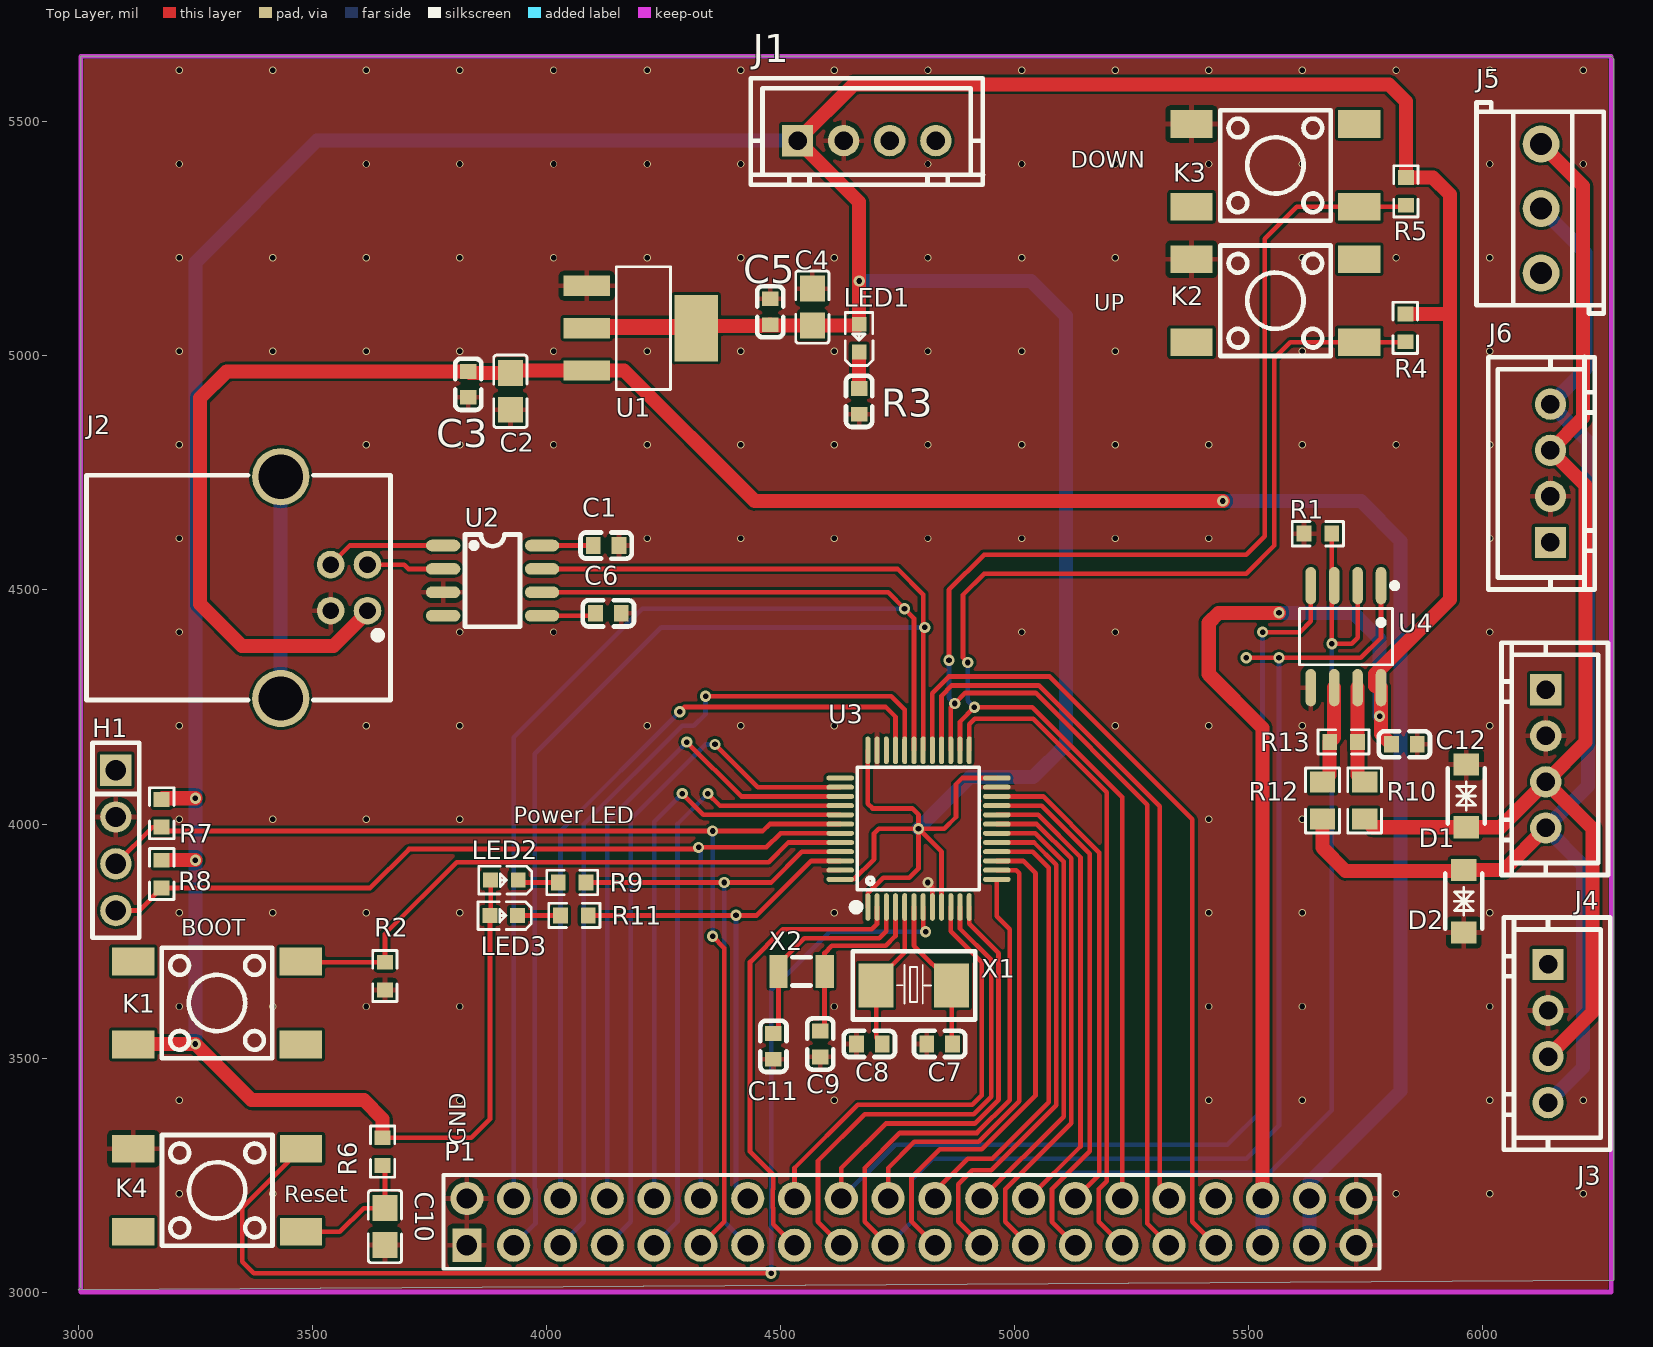
[diagram p0: Top Layer view]
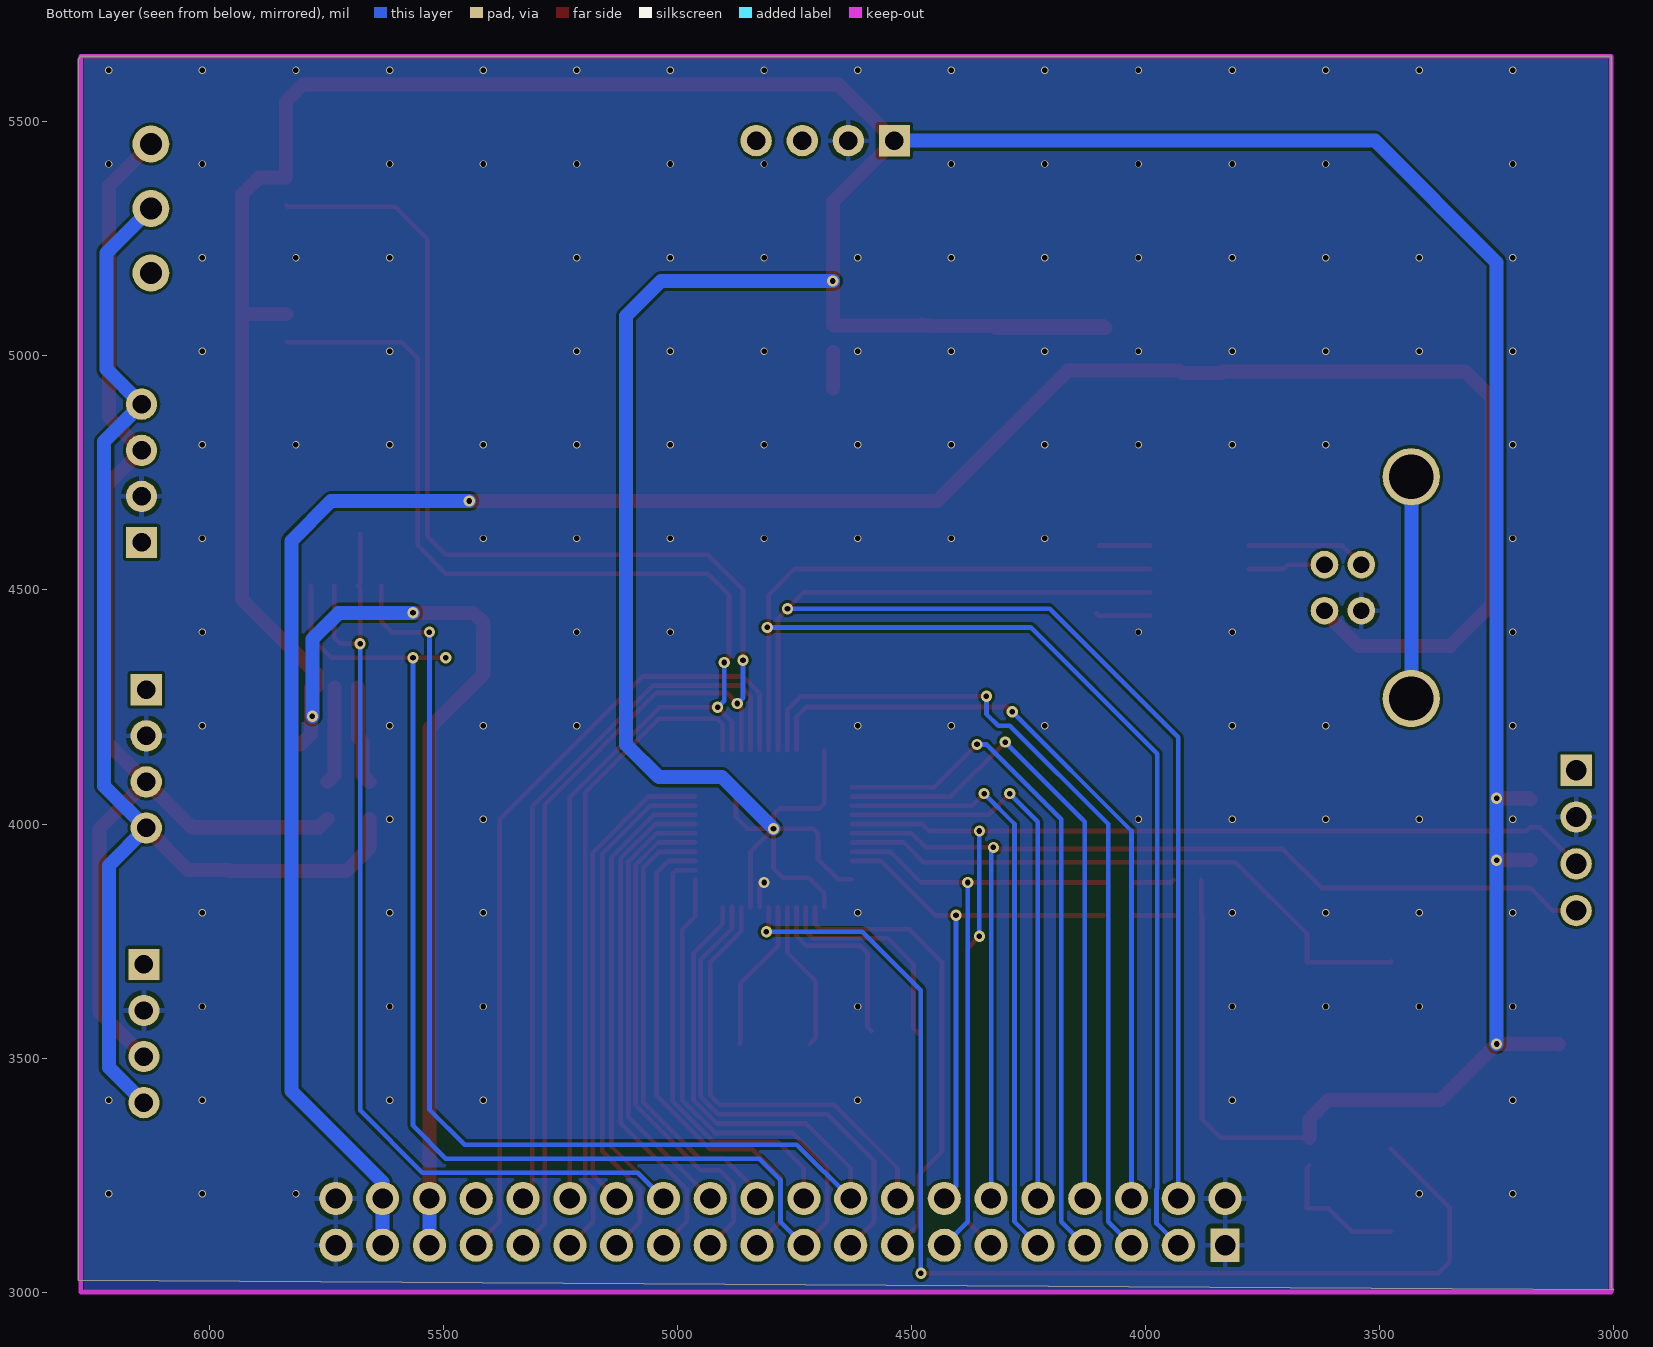
[diagram p1: Bottom Layer view, seen from below]
# Altium PCB MISC51869.pcbdoc
Units mil, origin at the board's own origin, x right, y up, seen from the top; angles counter-clockwise.
Board outline 3280 x 2635 mil, 2 copper layers (Top Layer, Bottom Layer); 48 components, 59 nets, 217 pads, 163 vias.

## Layer stack, top to bottom (the 12.6 mil dielectric is the usual default, probably not edited)
Top Solder Mask Layer: solder mask 0.4, Solder Resist, Dk 3.5
Top Layer: signal copper 1.4
Dielectric 1: surface 12.6, FR-4, Dk 4.8
Bottom Layer: signal copper 1.4
Bottom Solder Mask Layer: solder mask 0.4, Solder Resist, Dk 3.5

## Board outline
6280,3025 3000,3005 3005,3010 3005,5640 6275,5640 6280,5635

## Design rules (kind name [scope] priority, off if disabled: settings)
BoardOutlineClearance Clearance_1 [All] p2: genericclearance=6 ignorepadtopadclearanceinfootprint=FALSE except(0: Arc-SplitContinuation Track-SplitContinuation SMDPad-SplitContinuation THPad-SplitContinuation Via-SplitContinuation Fill-SplitContinuation Region-SplitContinuation Poly-SplitContinuation Text-SplitContinuation Hole-SplitContinuation; 6: Arc-OutlineEdge Track-OutlineEdge SMDPad-OutlineEdge THPad-OutlineEdge Via-OutlineEdge Fill-OutlineEdge Region-OutlineEdge Poly-OutlineEdge Text-OutlineEdge Hole-OutlineEdge SMDPad-CutoutEdge THPad-CutoutEdge Via-CutoutEdge Fill-CutoutEdge Region-CutoutEdge Poly-CutoutEdge Text-CutoutEdge; 6.9: Hole-CutoutEdge; 11.8: Arc-CutoutEdge Track-CutoutEdge)
Clearance [All] p1: gap=6 ignorepadtopadclearanceinfootprint=FALSE
DiffPairsRouting [All] p1: maxlimit=10 minlimit=6 mostfreqgap=6 toplayer_minwidth=15 toplayer_prefwidth=15 toplayer_maxwidth=15 toplayer_mingap=10 toplayer_prefgap=10 toplayer_maxgap=10 bottomlayer_minwidth=15 bottomlayer_prefwidth=15 bottomlayer_maxwidth=15 bottomlayer_mingap=10 bottomlayer_prefgap=10 bottomlayer_maxgap=10 maxuncoupledlength=10
HoleToHoleClearance ComponentClearance [All] p1: gap=0 allowstackedmicrovias=TRUE
Length netLength [All] p1: minlimit=0 maxlimit=0
MatchedLengths netLengthTolerance [All] p1: tolerance=1000
PlaneConnect PlaneConnect_1 [All] p1 off: planeconnectstyle=Direct reliefexpansion=20 reliefentries=4 reliefconductorwidth=10 reliefairgap=10
PlaneConnect [All] p2: planeconnectstyle=Relief reliefexpansion=20 reliefentries=4 reliefconductorwidth=10 reliefairgap=10
PolygonConnect [(InNet('GND'))] p1: connectstyle=Relief reliefconductorwidth=10 reliefentries=4 polygonreliefangle="90 Angle" airgapwidth=10 via.connectstyle=Relief via.reliefconductorwidth=10 via.reliefentries=4 via.polygonreliefangle="90 Angle" via.airgapwidth=10
RoutingVias [All] p1: holewidth=11.81 width=15.75 viastyle="Through Hole" minholewidth=11.81 minwidth=15.75 maxholewidth=39.37 maxwidth=50
SolderMaskExpansion [All] p1: expansion=4 istentingtop=FALSE
Width [All] p1: maxlimit=10 minlimit=10 preferedwidth=10 toplayer_minwidth=6 toplayer_maxwidth=100 toplayer_prefwidth=10 bottomlayer_minwidth=6 bottomlayer_maxwidth=100 bottomlayer_prefwidth=10
1 further rules are at their usual default settings.

## Components (designator, comment, footprint, x,y, rotation, side; value= is the part's Value field where it differs from the comment)
C1 "CC0603KRX7R9BB104" "C0603 - duplicate" 4127.56,4595 r0 top
C2 "CL21A106KAYNNNE" C0805 3923.06,4924.42 r90 top
C3 "CC0603KRX7R9BB104" "C0603 - duplicate" 3833.06,4939.42 r270 top
C4 "CL21A106KAYNNNE" C0805 4568.06,5104.42 r270 top
C5 "CC0603KRX7R9BB104" "C0603 - duplicate" 4478.06,5094.42 r270 top
C6 "CC0603KRX7R9BB104" "C0603 - duplicate" 4132.44,4450 r180 top
C7 "CL10C200JB8NNNC" C0603c20pf 4840,3530 r0 top
C8 "CL10C200JB8NNNC" C0603c20pf 4690,3530 r0 top
C9 "CL10C200JB8NNNC" C0603c20pf 4585,3530 r90 top
C10 "CL21A106KAYNNNE" C0805 3655,3140 r90 top
C11 "CL10C200JB8NNNC" C0603c20pf 4485,3525 r90 top
C12 "CC0603KRX7R9BB104" "C0603 - duplicate" 5833.07,4170.26 r0 top
D1 "SMF6.0CA_C2990473" 瞬态二极管 5965,4060 r90 top
D2 "SMF6.0CA_C2990473" 瞬态二极管 5960,3835 r90 top
H1 "PM254V-11-04-H85" 排母4p 3080,3965 r270 top
J1 "XH-4A" XH-4A 4684.21,5460 r0 top
J2 "USB-B-Female-90" USB-B_TH_USB-B-FEMALE-90 3525,4505 r270 top locked
J3 "XH-4A" XH-4A 6140,3552.35 r270 top
J4 "XH-4A" XH-4A 6135,4139.21 r270 top
J5 "KF350-3.5-3P" KF350-3.5-3P 6125,5315.01 r90 top
J6 "XH-4A" XH-4A 6145,4749.21 r90 top
K1 "KH-6X6X5H-STM" 按键 3296.15,3617.62 r0 top
K2 "KH-6X6X5H-STM" 复位按键 5557.37,5117.95 r180 top
K3 "KH-6X6X5H-STM" 复位按键 5557.37,5407.04 r180 top
K4 "KH-6X6X5H-STM" 复位按键 3296.56,3217.26 r180 top
LED1 "FC-D1608HGK-572C" LED0603-RD 4668.1,5038.06 r90 top
LED2 "FC-D1608HGK-572C" LED0603-RD 3910.16,3880.42 r180 top
LED3 "FC-D1608HGK-572C" LED0603-RD 3908.73,3804.57 r180 top
P1 "Header-Male-2.54_2x20" HDR-TH_40P-P2.54-V-M-R2-C20-S2.54 4780,3150 r0 top locked
R1 "0603WAF1002T5E" 电阻R0603 5648.07,4620.26 r180 top
R2 "0603WAF1002T5E" 电阻R0603 3655,3675 r270 top
R3 "0603WAF1001T5E" "C0603 - duplicate" 4668.1,4903.06 r90 top
R4 "0603WAF1002T5E" 电阻R0603 5835,5060 r270 top
R5 "0603WAF1002T5E" 电阻R0603 5836.09,5351.7 r270 top
R6 "0603WAF1002T5E" 电阻R0603 3650,3300 r270 top
R7 "0603WAF4701T5E" R06034.7k 3178,4023 r90 top
R8 "0603WAF4701T5E" R06034.7k 3178,3893 r90 top
R9 "0603WAF1001T5E" R06031k 4055,3875 r180 top
R10 "0805W8F200JT5E" R0805 5748.07,4050.26 r270 top
R11 "0603WAF1001T5E" R06031k 4059.58,3804.57 r180 top
R12 "0805W8F200JT5E" R0805 5658.07,4050.26 r270 top
R13 "0603WAF1200T5E" "R0603 - duplicate" 5703.07,4175.26 r0 top
U1 "AMS1117-3.3" SOT-223-3_L6.5-W3.4-P2.30-LS7.0-BR 4203.06,5059.42 r180 top
U2 "CH340N_C2977777" SOP-8_L4.9-W3.9-P1.27-LS6.0-BL 3885,4520 r270 top locked
U3 "STM32F103C8T6" LQFP-48_L7.0-W7.0-P0.50-LS9.0-BL 4795,3990 r0 top locked
U4 "SP3485EEN" 485SOP-8_L5.0-W4.0-P1.27-LS6.0-BL 5708.07,4400.26 r180 top
X1 "Q13FC1350000400" CRYSTAL-SMD_L5.0-W3.2 4785,3655 r180 top
X2 "X50328MSB2GI" FC-135R_L3.2-W1.5 4545,3685 r180 top

## Footprints (in the part's own frame and the unit in brackets; to place one, negate y for a bottom-side part, rotate by r counter-clockwise, add the part's x,y. Pads: shape width x height; smd on the part's side, far side on the other; paste and mask are expansions set on the pad)
485SOP-8_L5.0-W4.0-P1.27-LS6.0-BL [mil]
  oval 22.6x80.14 smd paste+2 mask+4: 1(-75,-108.97) 2(-25,-108.97) 3(25,-108.97) 4(75,-108.97) 5(75,108.97) 6(25,108.97) 7(-25,108.97) 8(-75,108.97)
  silkscreen extent -110,-115 99,60
"C0603 - duplicate" [mm]
  rect 0.8x0.9 smd paste+0.051 mask+0.102: 1(-0.7,0) 2(0.7,0)
  silkscreen extent -1.39,-0.71 1.39,0.71
C0603c20pf [mm]
  rect 0.8x0.9 smd paste+0.051 mask+0.102: 1(-0.7,0) 2(0.7,0)
  silkscreen extent -1.39,-0.71 1.39,0.71
C0805 [mm]
  rect 1.41x1.35 smd paste-100 mask+0.051: 1(-1,0) 2(1,0)
  silkscreen extent -1.96,-0.9 1.96,0.9
CRYSTAL-SMD_L5.0-W3.2 [mm]
  rect 1.9x2.4 smd paste+0.051 mask+0.102: 1(-2.05,0) 2(2.05,0)
  silkscreen extent -3.32,-1.85 3.33,1.85
FC-135R_L3.2-W1.5 [mm]
  rect 1x1.8 smd paste+0.051 mask+0.102: 1(-1.25,0) 2(1.25,0)
  silkscreen extent -0.51,-0.76 0.51,0.76
HDR-TH_40P-P2.54-V-M-R2-C20-S2.54 [mm]
  rect 1.575x1.8 hole 1.1 paste+0.051 mask+0.102: 1(-24.13,-1.27)
  round 1.8 hole 1.1 paste+0.051 mask+0.102: 2(-24.13,1.27) 3(-21.59,-1.27) 4(-21.59,1.27) 5(-19.05,-1.27) 6(-19.05,1.27) 7(-16.51,-1.27) 8(-16.51,1.27) 9(-13.97,-1.27) 10(-13.97,1.27) 11(-11.43,-1.27) 12(-11.43,1.27) 13(-8.89,-1.27) 14(-8.89,1.27) 15(-6.35,-1.27) 16(-6.35,1.27) 17(-3.81,-1.27) 18(-3.81,1.27) 19(-1.27,-1.27) 20(-1.27,1.27) 21(1.27,-1.27) 22(1.27,1.27) 23(3.81,-1.27) 24(3.81,1.27) 25(6.35,-1.27) 26(6.35,1.27) 27(8.89,-1.27) 28(8.89,1.27) 29(11.43,-1.27) 30(11.43,1.27) 31(13.97,-1.27) 32(13.97,1.27) 33(16.51,-1.27) 34(16.51,1.27) 35(19.05,-1.27) 36(19.05,1.27) 37(21.59,-1.27) 38(21.59,1.27) 39(24.13,-1.27) 40(24.13,1.27)
  silkscreen extent -25.4,-2.54 25.4,2.54
KF350-3.5-3P [mm]
  round 2 hole 1.2 paste+0.051 mask+0.102: 1(-3.5,0) 2(0,0) 3(3.5,0)
  silkscreen extent -5.7,-3.4 5.75,3.5
LED0603-RD [mm]
  rect 0.8x0.8 smd paste+0.051 mask+0.102: 1(-0.749,0) 2(0.749,0)
  silkscreen extent -1.49,-0.75 1.39,0.76
LQFP-48_L7.0-W7.0-P0.50-LS9.0-BL [mm]
  oval 0.27x1.5 smd paste+0 mask+0.05: 1(-2.75,-4.25) 2(-2.25,-4.25) 3(-1.75,-4.25) 4(-1.25,-4.25) 5(-0.75,-4.25) 6(-0.25,-4.25) 7(0.25,-4.25) 8(0.75,-4.25) 9(1.25,-4.25) 10(1.75,-4.25) 11(2.25,-4.25) 12(2.75,-4.25) 25(2.75,4.25) 26(2.25,4.25) 27(1.75,4.25) 28(1.25,4.25) 29(0.75,4.25) 30(0.25,4.25) 31(-0.25,4.25) 32(-0.75,4.25) 33(-1.25,4.25) 34(-1.75,4.25) 35(-2.25,4.25) 36(-2.75,4.25)
  oval 1.5x0.27 smd paste+0 mask+0.05: 13(4.25,-2.75) 14(4.25,-2.25) 15(4.25,-1.75) 16(4.25,-1.25) 17(4.25,-0.75) 18(4.25,-0.25) 19(4.25,0.25) 20(4.25,0.75) 21(4.25,1.25) 22(4.25,1.75) 23(4.25,2.25) 24(4.25,2.75) 37(-4.25,2.75) 38(-4.25,2.25) 39(-4.25,1.75) 40(-4.25,1.25) 41(-4.25,0.75) 42(-4.25,0.25) 43(-4.25,-0.25) 44(-4.25,-0.75) 45(-4.25,-1.25) 46(-4.25,-1.75) 47(-4.25,-2.25) 48(-4.25,-2.75)
  silkscreen extent -3.59,-4.46 3.3,3.34
"R0603 - duplicate" [mil]
  rect 31.75x34.02 smd paste-3937.01 mask+2: 1(-29.66,0) 2(29.66,0)
  silkscreen extent -55,-26 55,26
R0805 [mm]
  rect 1.133x1.377 smd paste-100 mask+0.051: 1(-1,0) 2(1,0)
  silkscreen extent -1.76,-0.92 1.76,0.92
R06031k [mil]
  rect 31.75x34.02 smd paste-3937.01 mask+2: 1(-29.66,0) 2(29.66,0)
  silkscreen extent -55,-26 55,26
R06034.7k [mil]
  rect 31.75x34.02 smd paste-3937.01 mask+2: 1(-29.66,0) 2(29.66,0)
  silkscreen extent -55,-26 55,26
SOP-8_L4.9-W3.9-P1.27-LS6.0-BL [mm]
  oval 0.63x1.865 smd paste+0.051 mask+0.102: 1(-1.905,-2.682) 2(-0.635,-2.682) 3(0.635,-2.682) 4(1.905,-2.682) 5(1.905,2.682) 6(0.635,2.682) 7(-0.635,2.682) 8(-1.905,2.682)
  silkscreen extent -2.5,-1.5 2.5,1.48
SOT-223-3_L6.5-W3.4-P2.30-LS7.0-BR [mm]
  rect 2.5x1.1 smd paste+0.051 mask+0.102: 1(2.97,-2.3) 2(2.97,0) 3(2.97,2.3)
  rect 2.34x3.6 smd paste+0.051 mask+0.102: 4(-2.97,0)
  silkscreen extent -1.57,-3.33 1.37,3.33
USB-B_TH_USB-B-FEMALE-90 [mm]
  round 1.5 hole 0.9 copper offset 0,0 paste+0.051 mask+0.102: 1(1.25,2.355) 2(-1.25,2.355) 3(-1.25,0.355) 4(1.25,0.355)
  round 3.1 hole 2.4 copper offset 0,0 paste+0.051 mask+0.102: 5(-6.02,-2.355) 6(6.02,-2.355)
  silkscreen extent -6.1,-12.89 6.1,3.61
XH-4A [mm]
  rect 1.7x1.7 hole 1 paste+0.051 mask+0.102: 1(-3.75,0)
  round 1.7 hole 1 paste+0.051 mask+0.102: 2(-1.25,0) 3(1.25,0) 4(3.75,0)
  silkscreen extent -6.3,-2.4 6.31,3.38
复位按键 [mm]
  rect 2.3x1.5 smd paste+0.051 mask+0.102: 1(-4.55,2.25) 2(4.55,2.25) 3(-4.55,-2.25) 4(4.55,-2.25)
  silkscreen extent -3,-3 3,3
按键 [mm]
  rect 2.3x1.5 smd paste+0.051 mask+0.102: 1(-4.55,-2.25) 2(4.55,-2.25) 3(-4.55,2.25) 4(4.55,2.25)
  silkscreen extent -3,-3 3,3
排母4p [mm]
  rect 1.7x1.7 hole 1.1 paste+0.051 mask+0.102: 1(-3.81,0)
  round 1.7 hole 1.1 paste+0.051 mask+0.102: 2(-1.27,0) 3(1.27,0) 4(3.81,0)
  silkscreen extent -5.29,-1.27 5.29,1.27
电阻R0603 [mil]
  rect 31.75x34.02 smd paste-3937.01 mask+2: 1(-29.66,0) 2(29.66,0)
  silkscreen extent -55,-26 55,26
瞬态二极管 [mm]
  rect 1.2x1.4 smd paste+0.051 mask+0.102: 1(-1.7,0) 2(1.7,0)
  silkscreen extent -1.5,-1 1.5,1

## Via types
v1: diameter 15.75, hole 11.8, Top Layer to Bottom Layer, 130 vias
v2: diameter 24.02, hole 12, Top Layer to Bottom Layer, 33 vias

## Nets (pads, with @x,y where several pads share a name; then routed paths per layer and width w, separated by ;. In a path a pad name is that pad's centre, name@x,y a point inside that pad or via, vN(x,y) a via of type N, cw(c..) or ccw(c..) an arc to the next point about the centre after c; other vN are vias at no path point)
$2N143: J2.5 J2.6 | length 474
  Bottom Layer w30: J2.6 J2.5
$2N144: J1.3
$2N145: J1.4
$2N146: C1.1 U2.8 | length 109.4
  Top Layer w10: U2.8 C1.1
$2N148: LED1.1 R3.2 | length 77.9
  Top Layer w30: R3.2 LED1.1
$2N149: P1.34
$2N151: C10.2 K4.1 R6.2 | length 293.3
  Top Layer w10: K4.1 3558.68,3128.68 3609.37,3179.37 C10.2 3655,3265.34 R6.2
$2N152: LED3.1 R11.2 | length 91.7
  Top Layer w10: LED3.1 R11.2
$2N154: R10.1 R13.2 U4.7 | length 208.2
  Top Layer w30: U4.7 5733.07,4175.6 R13.2 5732.73,4104.97 R10.1
$2N155: R12.1 R13.1 U4.6 | length 212
  Top Layer w30: R12.1 5673.41,4104.97 R13.1 5683.07,4184.92 U4.6
$2N156: LED2.1 R9.2 | length 87.9
  Top Layer w10: LED2.1 3945.08,3875 R9.2
A: D2.2 J3.4 J4.4 J5.2 J6.4 R12.2 | length 2712.2
  Top Layer w30: R12.2 5658.07,3949.32 5707.39,3900 5958.07,3900 D2.2 6045.37,3901.93 J4.4
  Bottom Layer w30: J5.2 6220,5220 6220,4971.86 J6.4 6225,4816.86 6225,4081.56 J4.4 6215,3911.56 6215,3479.7 J3.4
B: D1.1 J3.3 J4.3 J5.3 J6.3 R10.2 | length 2597.4
  Top Layer w30: R10.2 5765.89,3993.07 D1.1 6038.07,3993.07 J4.3 ; J5.3 6215,5362.8 6215,4868.42 J6.3 6220,4723.42 6220,4175 J4.3 ; J3.3 6235,3598.14 6235,3990 J4.3
BOOT0: K1.4 R2.1 U3.44 | length 1294.3
  Top Layer w10: K1.4 3476.83,3704.66 R2.1 3655,3765 3808.32,3918.32 4474.89,3918.32 4517.04,3960.47 U3.44
D+: J2.3 U2.1 | length 257.3
  Top Layer w10: J2.3 3579.76,4595 U2.1
D-: J2.2 U2.2 | length 165.5
  Top Layer w10: J2.2 3695.78,4554.22 3705,4545 U2.2
GND: C1.2 C2.1 C3.2 C4.1 C5.1 C6.1 C7.1 C8.1 C9.1 C10.1 C11.1 C12.2 D1.2 D2.1 H1.2 J1.2 J2.4 J3.2 J4.2 J6.2 K2.4 K3.4 K4.4 P1.1 P1.2 P1.39 P1.40 R1.2 R2.2 R3.1 U1.1 U2.3 U3.8 U3.23 U3.35 U3.47 U4.5 | length 56.3
  Top Layer w10: v2(4815,3875) 4824.53,3865.47 U3.8
  other v1: 3215.1,3210.1 3415.1,3210.1 5815.1,3210.1 6015.1,3210.1 6215.1,3210.1 3215.1,3410.1 3815.1,3410.1 4615.1,3410.1 5415.1,3410.1 5615.1,3410.1 6015.1,3410.1 6215.1,3410.1 3215.1,3610.1 3415.1,3610.1 3615.1,3610.1 3815.1,3610.1 4615.1,3610.1 5415.1,3610.1 5615.1,3610.1 6015.1,3610.1 3215.1,3810.1 3415.1,3810.1 3615.1,3810.1 3815.1,3810.1 4615.1,3810.1 5415.1,3810.1 5615.1,3810.1 6015.1,3810.1 3215.1,4010.1 3415.1,4010.1 3615.1,4010.1 3815.1,4010.1 4015.1,4010.1 5415.1,4010.1 5615.1,4010.1 3215.1,4210.1 3615.1,4210.1 3815.1,4210.1 4215.1,4210.1 4415.1,4210.1 4615.1,4210.1 5215.1,4210.1 5415.1,4210.1 5615.1,4210.1 6015.1,4210.1 3215.1,4410.1 3815.1,4410.1 4015.1,4410.1 5015.1,4410.1 5215.1,4410.1 6015.1,4410.1 3215.1,4610.1 4215.1,4610.1 4415.1,4610.1 4615.1,4610.1 4815.1,4610.1 5015.1,4610.1 5215.1,4610.1 5415.1,4610.1 6015.1,4610.1 3215.1,4810.1 3615.1,4810.1 3815.1,4810.1 4015.1,4810.1 4215.1,4810.1 4415.1,4810.1 4615.1,4810.1 4815.1,4810.1 5015.1,4810.1 5215.1,4810.1 5415.1,4810.1 5615.1,4810.1 5815.1,4810.1 6015.1,4810.1 3215.1,5010.1 3415.1,5010.1 3615.1,5010.1 3815.1,5010.1 4015.1,5010.1 4215.1,5010.1 4415.1,5010.1 4615.1,5010.1 4815.1,5010.1 5015.1,5010.1 5215.1,5010.1 5615.1,5010.1 6015.1,5010.1 3215.1,5210.1 3415.1,5210.1 3615.1,5210.1 3815.1,5210.1 4015.1,5210.1 4215.1,5210.1 4415.1,5210.1 4615.1,5210.1 4815.1,5210.1 5015.1,5210.1 5215.1,5210.1 5615.1,5210.1 5815.1,5210.1 6015.1,5210.1 3215.1,5410.1 3615.1,5410.1 3815.1,5410.1 4015.1,5410.1 4215.1,5410.1 4415.1,5410.1 4815.1,5410.1 5015.1,5410.1 5215.1,5410.1 5415.1,5410.1 5615.1,5410.1 6015.1,5410.1 6215.1,5410.1 3215.1,5610.1 3415.1,5610.1 3615.1,5610.1 3815.1,5610.1 4015.1,5610.1 4215.1,5610.1 4415.1,5610.1 4615.1,5610.1 4815.1,5610.1 5015.1,5610.1 5215.1,5610.1 5415.1,5610.1 5615.1,5610.1 5815.1,5610.1 6015.1,5610.1 6215.1,5610.1
NRST: K4.3 U3.7 | length 2474.9
  Top Layer w10: K4.3 3350,3180.16 3350,3065 3375,3040 v2(4480,3040) ; U3.7 4804.84,3775.16 v2(4810,3770)
  Bottom Layer w10: v2(4480,3040) 4480,3645 4605,3770 v2(4810,3770)
OSC32IN: C11.2 U3.3 X2.2 | length 463.7
  Top Layer w10: C11.2 4495.78,3563.34 X2.2 4495.78,3700.78 4551,3756 4711,3756 4726.1,3771.1 U3.3
OSC32OUT: C9.2 U3.4 X2.1 | length 399.1
  Top Layer w10: C9.2 4594.22,3566.78 X2.1 4594.22,3724.22 4610,3740 4725,3740 4745.79,3760.79 U3.4
OSCIN: C8.2 U3.5 X1.2 | length 323.5
  Top Layer w10: C8.2 4704.29,3543.27 X1.2 4704.29,3664.29 4765.47,3725.47 U3.5
OSCOUT: C7.2 U3.6 X1.1 | length 326.8
  Top Layer w10: U3.6 4785.16,3739.84 4865.71,3659.29 X1.1 4865.71,3531.85 C7.2
PA0: P1.16 U3.10 | length 959.3
  Top Layer w10: P1.16 4530,3265 4665,3400 4910,3400 4930,3420 4930,3705 4863.9,3771.1 U3.10
PA1: P1.17 U3.11 | length 1060.4
  Top Layer w10: P1.17 4580,3150 4580,3280 4680,3380 4912.63,3380 4950,3417.37 4950,3710 4883.58,3776.42 U3.11
PA4: P1.20 U3.14 | length 941.8
  Top Layer w10: P1.20 4730,3265 4786,3321 4923.37,3321 5010,3407.63 5010,3895 5003.58,3901.42 U3.14
PA5: P1.21 U3.15 | length 1071.7
  Top Layer w10: P1.21 4780,3150 4780,3245 4840,3305 4930,3305 5045,3420 5045,3895 5018.9,3921.1 U3.15
PA6: P1.22 U3.16 | length 962.7
  Top Layer w10: P1.22 4830,3215 4900,3285 4952.37,3285 5073,3405.63 5073,3906.49 5038.7,3940.79 U3.16
PA7: P1.23 U3.17 | length 1090.1
  Top Layer w10: P1.23 4880,3150 4880,3230 4910,3260 4950,3260 5089,3399 5089,3913.12 5041.65,3960.47 U3.17
PA8: P1.33 U3.29 | length 1749.4
  Top Layer w10: U3.29 4824.53,4279.53 4860,4315 5075,4315 5380,4010 5380,3150 P1.33
PA11: P1.5 U3.32 | length 1840.5
  Top Layer w10: v2(4340,4273.01) 4736.99,4273.01 4765.47,4244.53 U3.32
  Bottom Layer w10: P1.5 4080,3150 4080,4000 4290,4210 4315,4210 4340,4235 v2(4340,4273.01)
PA12: P1.6 U3.33 | length 1691.1
  Top Layer w10: v2(4285,4240) 4295,4250 4725,4250 4745.79,4229.21 U3.33
  Bottom Layer w10: P1.6 4030,3985 v2(4285,4240)
PA15: P1.7 U3.38 | length 1482.5
  Top Layer w10: v2(4360,4170) 4451.42,4078.58 U3.38
  Bottom Layer w10: P1.7 4180,3150 4180,4010 4340,4170 v2(4360,4170)
  other v2: 4360,4170
PB0: P1.24 U3.18 | length 959.9
  Top Layer w10: P1.24 5105,3375 5105,3919.75 5044.59,3980.16 U3.18
PB1: P1.25 U3.19 | length 1094.6
  Top Layer w10: U3.19 5047.53,3999.84 5121,3926.37 5121,3361 4980,3220 4980,3150 P1.25
PB2: P1.26 R1.1 U3.20 U4.2 U4.3 | length 3125.1
  Top Layer w10: U3.20 5050.47,4019.53 5141,3929 5141,3311 P1.26 ; R1.1 5677.73,4514.57 U4.3 5678.07,4504.23 v2(5678.07,4385.26) 5720.26,4385.26 5733.07,4398.07 U4.2
  Bottom Layer w10: P1.26 5085,3255 5545,3255 5678.07,3388.07 v2(5678.07,4385.26)
PB3: P1.8 U3.39 | length 1421.2
  Top Layer w10: v2(4300,4175) 4416.1,4058.9 U3.39
  Bottom Layer w10: P1.8 4130,4005 v2(4300,4175)
PB4: P1.9 U3.40 | length 1306
  Top Layer w10: v2(4345,4065) 4370.79,4039.21 U3.40
  Bottom Layer w10: P1.9 4280,3150 4280,4000 v2(4345,4065)
PB5: P1.10 U3.41 | length 1246.4
  Top Layer w10: v2(4290,4065) 4335.47,4019.53 U3.41
  Bottom Layer w10: P1.10 4230,4005 v2(4290,4065)
PB8: P1.13 R9.1 U3.45 | length 1366
  Top Layer w10: R9.1 v2(4380,3875) 4480,3875 4545.79,3940.79 U3.45
  Bottom Layer w10: v2(4380,3875) 4380,3150 P1.13
PB9: P1.14 R11.1 U3.46 | length 1202.1
  Top Layer w10: R11.1 4449.57,3804.57 4566.1,3921.1 U3.46
  Bottom Layer w10: v2(4405,3805) 4405,3225 P1.14
PB10: P1.27 U3.21 | length 1131.9
  Top Layer w10: U3.21 5058.16,4039.21 5161,3936.37 5161,3301 5080,3220 5080,3150 P1.27
PB11: P1.28 U3.22 | length 1028.5
  Top Layer w10: U3.22 5061.1,4058.9 5181,3939 5181,3251 P1.28
PB12: P1.29 U3.25 | length 1415.3
  Top Layer w10: U3.25 4903.27,4213.27 4915,4225 5040,4225 5197,4068 5197,3237 5180,3220 5180,3150 P1.29
PB15: P1.32 U3.28 | length 1544.6
  Top Layer w10: U3.28 4844.21,4274.21 4866,4296 5051.63,4296 5310,4037.63 5310,3220 P1.32
PC13: P1.15 U3.2 | length 986.7
  Top Layer w10: P1.15 4484.67,3145.33 4484.67,3179.67 4483.57,3180.77 4483.57,3219.23 4484.67,3220.33 4484.67,3250.33 4435,3300 4435,3705 4505,3775 4695,3775 4706.42,3786.42 U3.2
RXD1: P1.4 U2.6 U3.31 | length 3033.8
  Top Layer w10: U2.6 4730,4495 v2(4765,4460) 4785.16,4439.84 U3.31
  Bottom Layer w10: P1.4 3930,4185 4205,4460 v2(4765,4460)
RXD2: P1.19 U3.13 U4.1 | length 3455.7
  Top Layer w10: P1.19 4680,3150 4680,3265 4755,3340 4919.75,3340 4990,3410.25 4990,3775 4962.32,3802.68 U3.13 ; v2@5490.43,4359.57 v2(5495,4355) v2(5565,4355) 5740,4355 5783.07,4398.07 U4.1
  Bottom Layer w10: P1.19 4780,3150 4780,3240 4825,3285 5495,3285 5565,3355 v2(5565,4355)
SCL1: H1.3 P1.11 R7.1 U3.42 | length 2505.8
  Top Layer w10: H1.3 3158.34,3993.34 R7.1 3186.33,3985 v2(4355,3985) 4462.1,3985 4476.94,3999.84 U3.42 ; P1.11 4380,3150 4380,3735 v2(4355,3760)
  Bottom Layer w10: v2(4355,3760) v2(4355,3985)
SDA1: H1.4 P1.12 R8.1 U3.43 | length 2368.2
  Top Layer w10: H1.4 3129.66,3815 R8.1 3623.34,3863.34 3706.54,3946.54 4321.54,3946.54 v2(4325,3950) 4470,3950 4500.16,3980.16 U3.43
  Bottom Layer w10: v2(4325,3950) 4330,3945 P1.12
SWCLK: U3.37
SWDIO: U3.34
SWDOWN: K3.1 P1.31 R5.2 U3.27 | length 3519.9
  Top Layer w10: v2(4860,4350) 4860,4500 4935,4575 5495,4575 5535,4615 5535,5250 5603.46,5318.46 K3.1 5832.51,5318.46 R5.2 ; U3.27 4863.9,4248.9 v2(4872.47,4257.47) 4895,4280 5045,4280 5283.57,4041.43 5283.57,3146.43 P1.31
  Bottom Layer w10: v2(4860,4350) 4860,4269.94 v2(4872.47,4257.47)
SWUP: K2.1 P1.30 R4.2 U3.26 | length 3011.3
  Top Layer w10: U3.26 4883.58,4218.58 v2(4914.38,4249.38) 5038.24,4249.38 5230,4057.63 P1.30 ; v2(4900,4345) 4890,4355 4890,4490 4935,4535 5495,4535 5555,4595 5555,4995 5589.36,5029.36 K2.1 5834.02,5029.36 R4.2
  Bottom Layer w10: v2(4900,4345) 4900,4263.77 v2(4914.38,4249.38)
TXD1: P1.3 U2.7 U3.30 | length 3184.6
  Top Layer w10: U2.7 4750,4545 4804.84,4490.16 U3.30
  Bottom Layer w10: P1.3 3976.43,3146.43 3976.43,3219.23 3975,3220.67 3975,4150 4245,4420 v2(4808.17,4420)
TXD2: P1.18 U3.12 U4.4 | length 3086.8
  Top Layer w10: P1.18 4630,3265 4725,3360 4915.25,3360 4966,3410.75 4966,3724 4903.27,3786.73 U3.12 ; v2(5530,4410) 5610,4410 5633.07,4433.07 U4.4
  Bottom Layer w10: P1.18 4745,3315 5455,3315 5530,3390 v2(5530,4410)
VCC3V: H1.1
VCC3V3: C4.2 C5.2 C12.1 J1.1 K1.1 LED1.2 LED2.2 LED3.2 P1.35 P1.36 R4.1 R5.1 R6.1 R7.2 R8.2 U1.2 U1.4 U3.1 U3.9 U3.24 U3.36 U3.48 U4.8 | length 13761.7
  Top Layer w10: R6.1 3839.66,3329.66 3879.24,3369.24 LED3.2 3880.68,3806 LED2.2 ; U3.48 4656.73,3881.73 4700,3925 4700,3980 4710,3990 v2(4795,3990) ; U3.1 4686.73,3851.73 4720,3885 4775,3885 4795,3905 v2(4795,3990) ; U3.36 4686.73,4043.27 4696.73,4033.27 4781.73,4033.27 4795,4020 v2(4795,3990) ; U3.9 4844.21,3940.79 v2(4795,3990) ; U3.24 4888.27,4098.27 4875,4085 4875,4015 4850,3990 v2(4795,3990)
  Top Layer w30: K1.1 3117.98,3530 v2(3250,3530) 3370,3410 3610,3410 3650,3370 R6.1 ; R8.2 v2(3250,3922.66) ; R7.2 3180.34,4055 v2(3250,4055) ; U1.4 U1.2 4091.14,5064.42 4457.65,5064.42 4458.28,5065.05 C5.2@4479.87,5065.05 ; C5.2 C5.2@4479.87,5065.05 ; P1.36 5530,4205 5415,4320 5415,4430 5436.21,4451.21 v2(5565,4451.21) ; 5770,4295 5770,4320 5930,4480 5930,5089.1 ; U4.8 5783.07,4192.7 C12.1 ; R4.1 5929.44,5089.66 5930,5089.1 ; C5.2@4479.87,5065.05 C4.2 4665.59,5065.05 LED1.2 v2(4668.09,5160) 4668.09,5328.47 J1.1 4656.56,5580 5800,5580 5836.09,5543.91 R5.1 5893.64,5381.36 5930,5345 5930,5089.1
  Bottom Layer w30: v2(3250,3530) v2(3250,3922.66) v2(3250,4055) 3250,5200 3510,5460 J1.1 ; v2(4668.09,5160) 5035,5160 5110,5085 5110,4170 5040,4100 4905,4100 v2(4795,3990) ; P1.35 P1.36 ; v2(5565,4451.21) 5723.79,4451.21 5780,4395 v2(5780,4230)
VCC5V: C2.2 C3.1 J2.1 P1.37 P1.38 U1.3 | length 5196.7
  Top Layer w30: J2.1 3617.72,4452.72 3545,4380 3350,4380 3260,4470 3260,4910 3316.98,4966.98 C3.1 3836.25,4963.79 C2.2 3928.14,4968.87 U1.3 4166.13,4968.87 4445,4690 v2(5445,4690)
  Bottom Layer w30: v2(5445,4690) 5740,4690 5825,4605 5825,3430 5630,3235 P1.38 P1.37
VCC5V5: C6.2 U2.5 | length 116.3
  Top Layer w10: U2.5 4099.88,4445 C6.2
pads on no net: J3.1 J4.1 J5.1 J6.1 K1.2 K1.3 K2.2 K2.3 K3.2 K3.3 K4.2 U2.4

## Polygon pours and split planes (outlines as drawn)
GND on Top Layer (solid, remove dead copper, pour order 0): 3005,5640 3005,3000 6275,3000 6275,5640
GND on Bottom Layer (solid, remove dead copper, pour order 2): 3005,5640 3005,3000 6275,3000 6275,5640

## Keep-outs
Board Outline Layer:
  lines w10: 3005,3000 3005,5640 6275,5640 6275,3000 3005,3000

## Silkscreen, mask and mechanical layers (free items; w line width, h text height)
Top Silkscreen Layer:
  text "DOWN" at 5120,5390 h60
  text "UP" at 5170,5085 h60
  text "Power LED" at 3930,3990 h60
  text "BOOT" at 3220,3750 h60
  text "GND" at 3839.33,3315 h60 r90
  text "Reset" at 3440,3180 h60